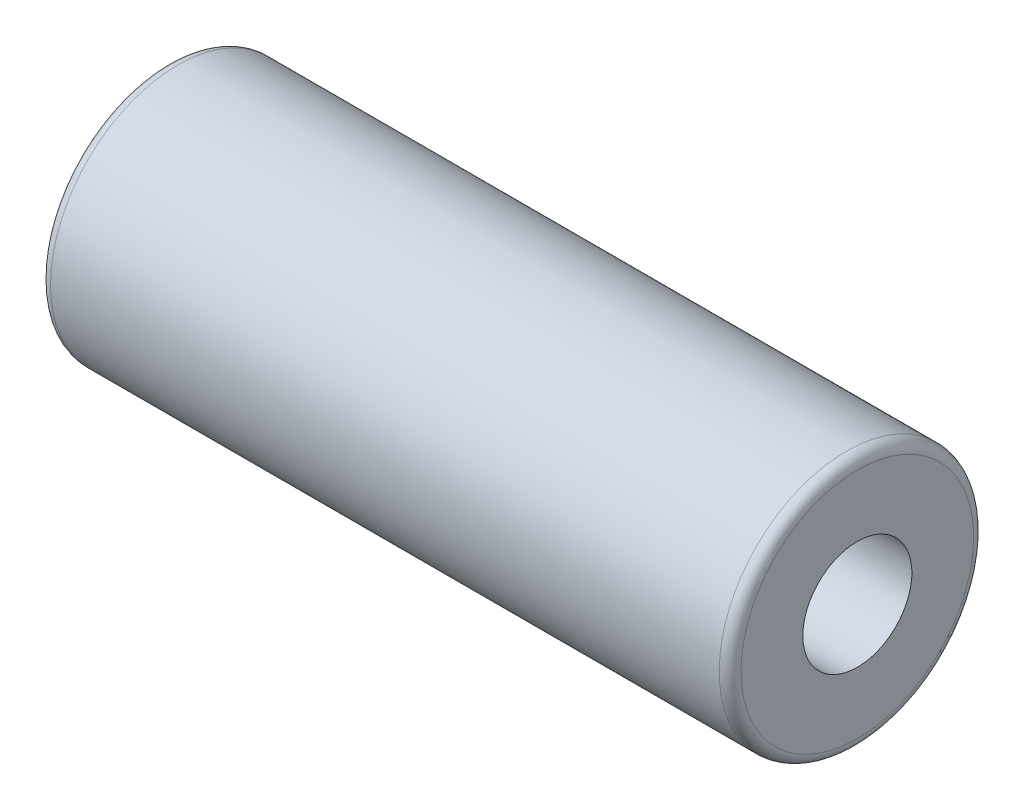
SolidWorks part; units mm, degrees
ref_plane "Front Plane" through (0, 0, 0) normal (0, 0, 1) x (1, 0, 0)
ref_plane "Top Plane" through (0, 0, 0) normal (0, 1, 0) x (1, 0, 0)
ref_plane "Right Plane" through (0, 0, 0) normal (1, 0, 0) x (0, 0, -1)
sketch "Sketch1" plane through (0, 0, 0) normal (0, 0, 1) x (1, 0, 0)
  line L0 (0, 1.5) -> (19, 1.5)
  line L1 (19, 1.5) -> (19, 3.2)
  line L2 (18.7, 3.5) -> (0.3, 3.5)
  line L3 (0, 3.2) -> (0, 1.5)
  line L4 (50, 0) -> (-50, 0) construction
  arc A0 (19, 3.2) -> (18.7, 3.5) centre (18.7, 3.2) ccw
  arc A1 (0.3, 3.5) -> (0, 3.2) centre (0.3, 3.2) ccw
revolve "Revolve1" add sketch "Sketch1" angle 360 about L4
